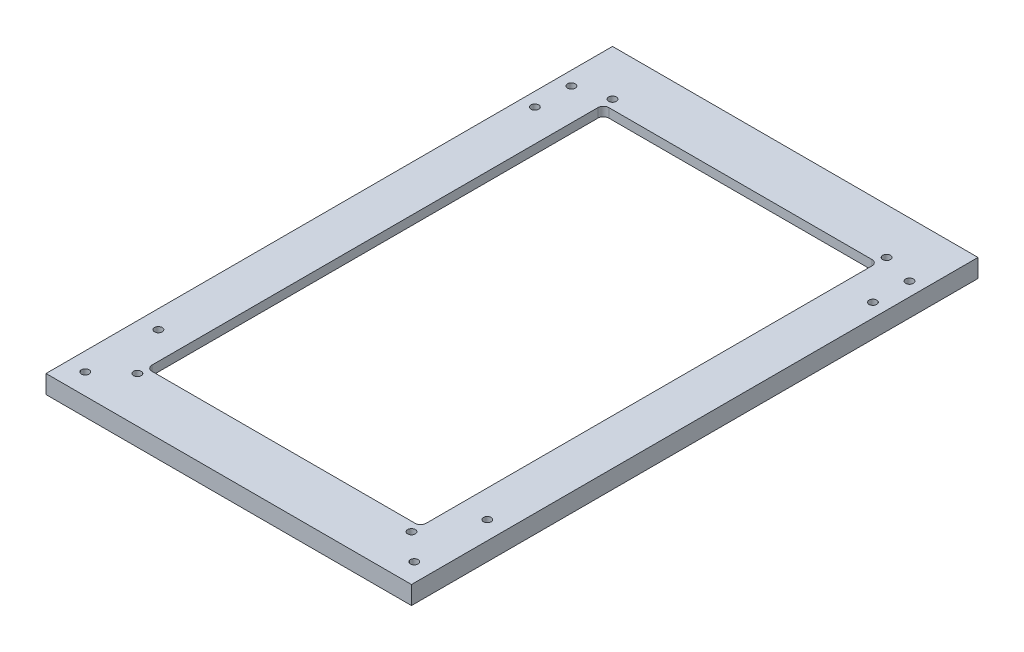
from build123d import *

# Parameters (mm, degrees)
SKETCH_1_W          = 200
SKETCH_1_H          = 310
EXTRUDE_1_DEPTH     = 5
SKETCH_2_W          = 150
SKETCH_2_H          = 250
CUT_EXTRUDE_1_DEPTH = 185.729532019
FILLET_1_R          = 3
SKETCH_13_W         = 170
SKETCH_13_H         = 280
CUT_EXTRUDE_2_DEPTH = 5
HOLE_WIZARD_M5_4_D  = 4.2
FILLET_2_R          = 5
HOLE_WIZARD_M5_5_D  = 4.2
HOLE_WIZARD_M5_6_D  = 4.2


with BuildPart() as part:
    # 草图1 → 凸台-拉伸1 (new, symmetric)
    with BuildSketch(Plane(origin=(0, 0, 0), x_dir=(1, 0, 0), z_dir=(0, 1, 0))):
        Rectangle(SKETCH_1_W, SKETCH_1_H)
    extrude(amount=EXTRUDE_1_DEPTH, both=True)

    # 草图2 → 切除-拉伸1 (cut, through all)
    with BuildSketch(Plane.XZ.offset(5)):
        Rectangle(SKETCH_2_W, SKETCH_2_H)
    extrude(amount=-CUT_EXTRUDE_1_DEPTH, mode=Mode.SUBTRACT)

    # 圆角1
    fillet_1_edges = [part.edges().sort_by_distance(p)[0] for p in [
        (75, 0, 125),
        (75, 0, -125),
        (-75, 0, -125),
        (-75, 0, 125),
    ]]
    fillet(fillet_1_edges, radius=FILLET_1_R)

    # 草图13 → 切除-拉伸2 (cut)
    with BuildSketch(Plane.XZ.offset(5)):
        Rectangle(SKETCH_13_W, SKETCH_13_H)
    extrude(amount=-CUT_EXTRUDE_2_DEPTH, mode=Mode.SUBTRACT)

    # M5 螺纹孔4 (through all)
    with Locations(Plane(origin=(0, 5, 0), x_dir=(1, 0, 0), z_dir=(0, 1, 0))):
        with Locations((92.5, 105), (92.5, 125), (-92.5, 105), (-92.5, 125)):
            Hole(HOLE_WIZARD_M5_4_D / 2)

    # 圆角2
    fillet_2_edges = [part.edges().sort_by_distance(p)[0] for p in [
        (85, -2.5, 140),
        (85, -2.5, -140),
        (-85, -2.5, -140),
        (-85, -2.5, 140),
    ]]
    fillet(fillet_2_edges, radius=FILLET_2_R)

    # M5 螺纹孔5 (through all)
    with Locations(Plane(origin=(0, 5, 0), x_dir=(1, 0, 0), z_dir=(0, 1, 0))):
        with Locations((-90, -103.5), (-90, -143.5), (90, -103.5), (90, -143.5)):
            Hole(HOLE_WIZARD_M5_5_D / 2)

    # M5 螺纹孔6 (through all)
    with Locations(Plane(origin=(0, 0, 0), x_dir=(-1, 0, 0), z_dir=(0, -1, 0))):
        with Locations((75, -130), (-75, -130), (75, 130), (-75, 130)):
            Hole(HOLE_WIZARD_M5_6_D / 2)


solid = part.part
